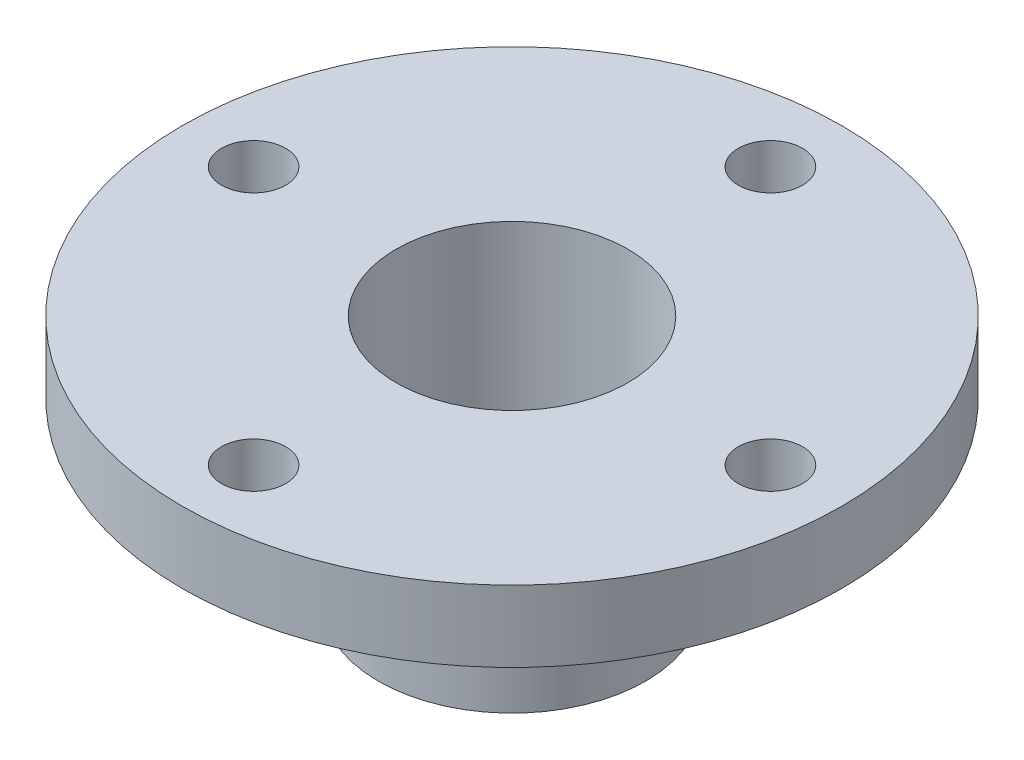
SolidWorks part; units mm, degrees
ref_plane "前视基准面" through (0, 0, 0) normal (0, 0, 1) x (1, 0, 0)
ref_plane "上视基准面" through (0, 0, 0) normal (0, 1, 0) x (1, 0, 0)
ref_plane "右视基准面" through (0, 0, 0) normal (1, 0, 0) x (0, 0, -1)
sketch "草图1" plane through (0, 0, 0) normal (0, 1, 0) x (1, 0, 0)
  circle A0 centre (0, 0) radius 32.5
  circle A1 centre (0, 0) radius 37.5
  dimension "D1" = 65
  dimension "D2" = 75
extrude "凸台-拉伸1" add sketch "草图1" along normal blind 50
sketch "草图2" plane through (0, 50, 0) normal (0, 1, 0) x (1, 0, 0)
  circle A0 centre (0, 0) radius 37.5
  circle A1 centre (0, 0) radius 92.5
  circle A2 centre (0, 0) radius 72.5 construction
  circle A3 centre (-72.5, 0) radius 9
  circle A4 centre (0, 72.5) radius 9
  circle A5 centre (72.5, 0) radius 9
  circle A6 centre (0, -72.5) radius 9
  circle A7 centre (0, 0) radius 37.5 construction
  point P23 (0, 0)
  dimension "D1" = 185
  dimension "D2" = 145
  dimension "D3" = 18
  dimension "D5" = 0
  dimension "D4" = 4
extrude "凸台-拉伸2" add sketch "草图2" along normal blind 20
sketch "草图3" plane through (0, 50, 0) normal (0, 1, 0) x (1, 0, 0)
  circle A1 centre (0, 0) radius 37.5
  circle A2 centre (0, 0) radius 37.5
  dimension "D1" = 0
extrude "凸台-拉伸3" add sketch "草图3" along normal up to surface (20 mm away) up to face at (72.5, 70, 9)
sketch "草图4" plane through (0, 50, 0) normal (0, -1, 0) x (1, 0, 0)
  circle A1 centre (0, 0) radius 32.5
  circle A2 centre (0, 0) radius 32.5
  dimension "D1" = 0
extrude "切除-拉伸1" cut sketch "草图4" against normal through all
